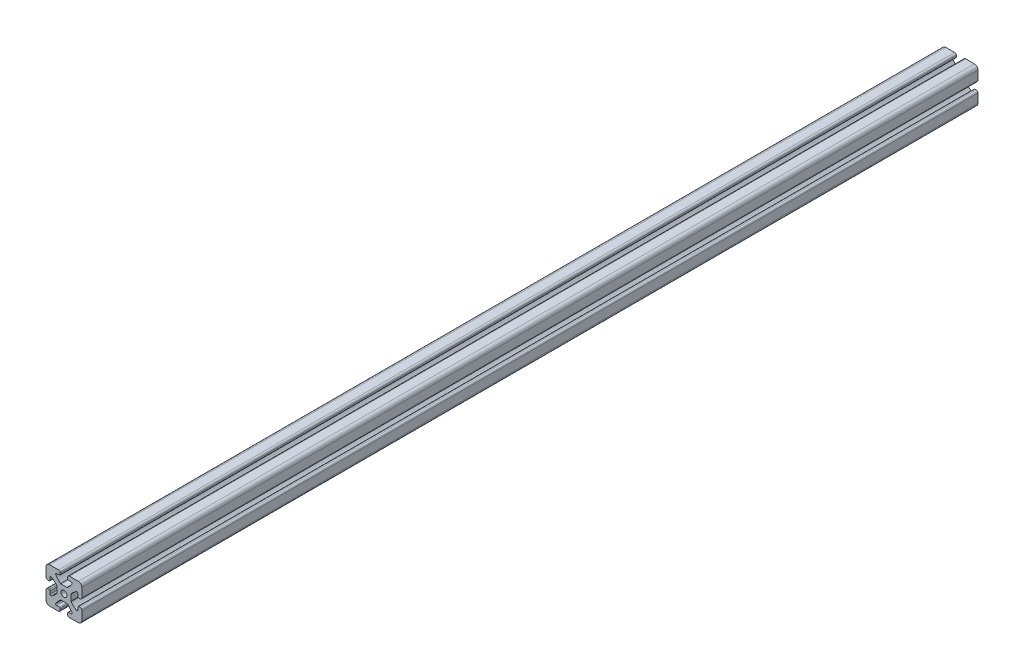
SolidWorks part; units mm, degrees
ref_plane "Front Plane" through (0, 0, 0) normal (0, 0, 1) x (1, 0, 0)
ref_plane "Top Plane" through (0, 0, 0) normal (0, 1, 0) x (1, 0, 0)
ref_plane "Right Plane" through (0, 0, 0) normal (1, 0, 0) x (0, 0, -1)
sketch "Sketch1" plane through (0, 0, 0) normal (0, 0, 1) x (1, 0, 0)
  line L0 (-75.7088, -20.1458) -> (-72.5526, -20.1458)
  line L1 (-70.701, -12.3958) -> (-67.4526, -12.3958)
  line L2 (-96.3499, -4.6458) -> (-39.5519, -4.6458) construction
  line L3 (-87.4526, 11.3542) -> (-87.4526, 1.3542)
  line L4 (-83.4526, -24.6458) -> (-73.5526, -24.6458)
  line L5 (-87.4526, -10.6458) -> (-87.4526, -20.6458)
  line L6 (-83.4526, 15.3542) -> (-73.4526, 15.3542)
  line L7 (-47.4526, -10.6458) -> (-47.4526, -20.6458)
  line L8 (-51.4526, -24.6458) -> (-61.4526, -24.6458)
  line L9 (-59.1964, -20.1458) -> (-62.4526, -20.1458)
  line L10 (-51.4526, 15.3542) -> (-61.4526, 15.3542)
  line L11 (-47.4526, 11.3542) -> (-47.4526, 1.3542)
  line L12 (-64.2043, -12.3958) -> (-67.4526, -12.3958)
  line L13 (-71.5526, -21.1458) -> (-71.5526, -22.6458)
  line L14 (-63.3526, -21.1458) -> (-63.3526, -22.6458)
  line L15 (-50.9526, -8.7458) -> (-49.4526, -8.7458)
  line L16 (-51.9526, -12.902) -> (-51.9526, -9.7458)
  line L17 (-59.7026, -7.8942) -> (-59.7026, -4.6458)
  line L18 (-50.9526, -0.5458) -> (-49.4526, -0.5458)
  line L19 (-51.9526, 3.6104) -> (-51.9526, 0.3542)
  line L20 (-59.7026, -1.3975) -> (-59.7026, -4.6458)
  line L21 (-63.3526, 11.8542) -> (-63.3526, 13.3542)
  line L22 (-59.1964, 10.8542) -> (-62.3526, 10.8542)
  line L23 (-63.8526, 3.1042) -> (-67.4526, 3.1042)
  line L24 (-71.5526, 11.8542) -> (-71.5526, 13.3542)
  line L25 (-75.7088, 10.8542) -> (-72.4526, 10.8542)
  line L26 (-71.0526, 3.1042) -> (-67.4526, 3.1042)
  line L27 (-83.9526, -0.5458) -> (-85.4526, -0.5458)
  line L28 (-82.9526, 3.6104) -> (-82.9526, 0.4542)
  line L29 (-75.2026, -1.3975) -> (-75.2026, -4.6458)
  line L30 (-83.9526, -8.7458) -> (-85.4526, -8.7458)
  line L31 (-82.9526, -12.902) -> (-82.9526, -9.6458)
  line L32 (-75.2026, -7.8942) -> (-75.2026, -4.6458)
  line L33 (-67.4526, 16.4313) -> (-67.4526, -26.9314) construction
  arc A0 (-71.3325, -12.6205) -> (-76.5532, -18.6101) centre (-55.648, -31.5616) ccw
  arc A1 (-76.5532, -18.6101) -> (-75.7088, -20.1458) centre (-75.7088, -19.1458) ccw
  arc A2 (-70.701, -12.3958) -> (-71.3325, -12.6205) centre (-70.701, -13.3958) ccw
  arc A3 (-83.4526, 15.3542) -> (-87.4526, 11.3542) centre (-83.4526, 11.3542) ccw
  arc A4 (-87.4526, -20.6458) -> (-83.4526, -24.6458) centre (-83.4526, -20.6458) ccw
  arc A6 (-63.5727, -12.6205) -> (-64.2043, -12.3958) centre (-64.2043, -13.3958) ccw
  arc A7 (-58.352, -18.6101) -> (-63.5727, -12.6205) centre (-79.2572, -31.5616) ccw
  arc A8 (-59.1964, -20.1458) -> (-58.352, -18.6101) centre (-59.1964, -19.1458) ccw
  arc A9 (-51.4526, -24.6458) -> (-47.4526, -20.6458) centre (-51.4526, -20.6458) ccw
  arc A10 (-47.4526, 11.3542) -> (-51.4526, 15.3542) centre (-51.4526, 11.3542) ccw
  circle A11 centre (-67.4526, -4.6458) radius 3.4
  arc A12 (-71.5526, -21.1458) -> (-72.5526, -20.1458) centre (-72.5526, -21.1458) ccw
  arc A13 (-73.5526, -24.6458) -> (-71.5526, -22.6458) centre (-73.5526, -22.6458) ccw
  arc A14 (-62.3526, -20.1458) -> (-63.3526, -21.1458) centre (-62.3526, -21.1458) ccw
  arc A15 (-63.3526, -22.6458) -> (-61.3526, -24.6458) centre (-61.3526, -22.6458) ccw
  arc A16 (-59.7026, -7.8942) -> (-59.478, -8.5257) centre (-58.7026, -7.8942) ccw
  arc A17 (-59.478, -8.5257) -> (-53.4884, -13.7464) centre (-40.5368, 7.1588) ccw
  arc A18 (-53.4884, -13.7464) -> (-51.9526, -12.902) centre (-52.9526, -12.902) ccw
  arc A19 (-50.9526, -8.7458) -> (-51.9526, -9.7458) centre (-50.9526, -9.7458) ccw
  arc A20 (-47.4526, -10.7458) -> (-49.4526, -8.7458) centre (-49.4526, -10.7458) ccw
  arc A21 (-59.478, -0.7659) -> (-59.7026, -1.3975) centre (-58.7026, -1.3975) ccw
  arc A22 (-53.4884, 4.4548) -> (-59.478, -0.7659) centre (-40.5368, -16.4504) ccw
  arc A23 (-51.9526, 0.4542) -> (-50.9526, -0.5458) centre (-50.9526, 0.4542) ccw
  arc A24 (-49.4526, -0.5458) -> (-47.4526, 1.4542) centre (-49.4526, 1.4542) ccw
  arc A25 (-51.9526, 3.6104) -> (-53.4884, 4.4548) centre (-52.9526, 3.6104) ccw
  arc A26 (-64.2043, 3.1042) -> (-63.5727, 3.3289) centre (-64.2043, 4.1042) ccw
  arc A27 (-63.5727, 3.3289) -> (-58.352, 9.3184) centre (-79.2572, 22.27) ccw
  arc A28 (-58.352, 9.3184) -> (-59.1964, 10.8542) centre (-59.1964, 9.8542) ccw
  arc A29 (-63.3526, 11.8542) -> (-62.3526, 10.8542) centre (-62.3526, 11.8542) ccw
  arc A30 (-61.3526, 15.3542) -> (-63.3526, 13.3542) centre (-61.3526, 13.3542) ccw
  arc A31 (-71.3325, 3.3289) -> (-70.701, 3.1042) centre (-70.701, 4.1042) ccw
  arc A32 (-76.5532, 9.3184) -> (-71.3325, 3.3289) centre (-55.648, 22.27) ccw
  arc A33 (-72.5526, 10.8542) -> (-71.5526, 11.8542) centre (-72.5526, 11.8542) ccw
  arc A34 (-71.5526, 13.3542) -> (-73.5526, 15.3542) centre (-73.5526, 13.3542) ccw
  arc A35 (-75.7088, 10.8542) -> (-76.5532, 9.3184) centre (-75.7088, 9.8542) ccw
  arc A36 (-75.2026, -1.3975) -> (-75.4273, -0.7659) centre (-76.2026, -1.3975) ccw
  arc A37 (-75.4273, -0.7659) -> (-81.4169, 4.4548) centre (-94.3684, -16.4504) ccw
  arc A38 (-81.4169, 4.4548) -> (-82.9526, 3.6104) centre (-81.9526, 3.6104) ccw
  arc A39 (-83.9526, -0.5458) -> (-82.9526, 0.4542) centre (-83.9526, 0.4542) ccw
  arc A40 (-87.4526, 1.4542) -> (-85.4526, -0.5458) centre (-85.4526, 1.4542) ccw
  arc A41 (-75.4273, -8.5257) -> (-75.2026, -7.8942) centre (-76.2026, -7.8942) ccw
  arc A42 (-81.4169, -13.7464) -> (-75.4273, -8.5257) centre (-94.3684, 7.1588) ccw
  arc A43 (-82.9526, -9.7458) -> (-83.9526, -8.7458) centre (-83.9526, -9.7458) ccw
  arc A44 (-85.4526, -8.7458) -> (-87.4526, -10.7458) centre (-85.4526, -10.7458) ccw
  arc A45 (-82.9526, -12.902) -> (-81.4169, -13.7464) centre (-81.9526, -12.902) ccw
extrude "Boss-Extrude1" add sketch "Sketch1" along normal blind 1000 contours A45 L31 A43 L30 A44 L5 A4 L4 A13 L13 A12 L0 A1 A0 A2 L1 L12 A6 A7 A8 L9 A14 L14 A15 L8 A9 L7 A20 L15 A19 L16 A18 A17 A16 L17 L20 A21 A22 A25 L19 A23 L18 A24 L11 A10 L10 A30 L21 A29 L22 A28
